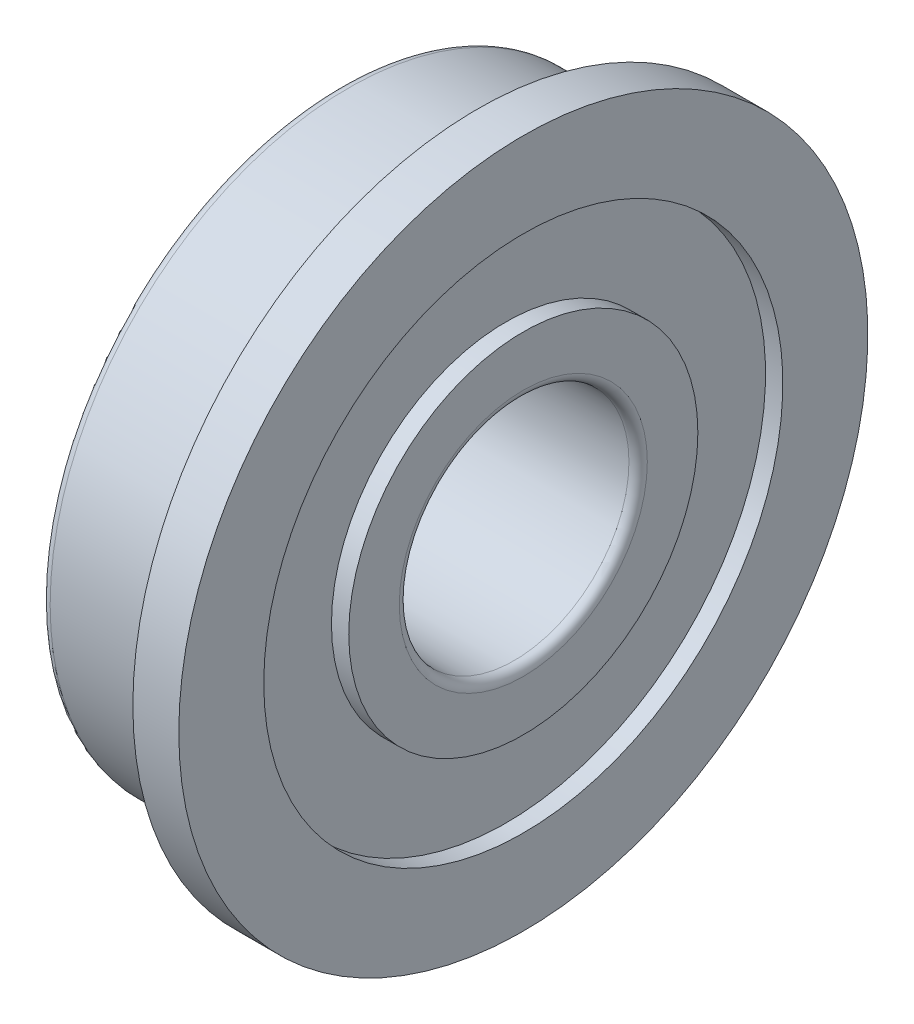
from build123d import *


with BuildPart() as part:
    # Sketch1 → Revolve1 (revolve)
    with BuildSketch(Plane.XY, mode=Mode.PRIVATE) as revolve1_sk:
        with BuildLine():
            Line((0, 6.3), (0, 5.65))
            Line((0, 5.65), (0.3765, 5.65))
            Line((0.3765, 5.65), (0.3765, 3.8))
            Line((0.3765, 3.8), (0, 3.8))
            Line((0, 3.8), (0, 2.7))
            ThreePointArc((0, 2.7), (0.058578644, 2.558578644), (0.2, 2.5))
            Line((0.2, 2.5), (3.8, 2.5))
            ThreePointArc((3.8, 2.5), (3.941421356, 2.558578644), (4, 2.7))
            Line((4, 2.7), (4, 3.8))
            Line((4, 3.8), (3.6235, 3.8))
            Line((3.6235, 3.8), (3.6235, 5.65))
            Line((3.6235, 5.65), (4, 5.65))
            Line((4, 5.65), (4, 7.5))
            Line((4, 7.5), (3, 7.5))
            Line((3, 7.5), (3, 6.7))
            ThreePointArc((3, 6.7), (3.141421356, 6.358578644), (2.8, 6.5))
            Line((2.8, 6.5), (0.2, 6.5))
            ThreePointArc((0.2, 6.5), (0.058578644, 6.441421356), (0, 6.3))
        make_face()
    revolve(revolve1_sk.sketch.rotate(Axis((13, 0, 0), (-1, 0, 0)), 270), axis=Axis((13, 0, 0), (-1, 0, 0)))


solid = part.part
